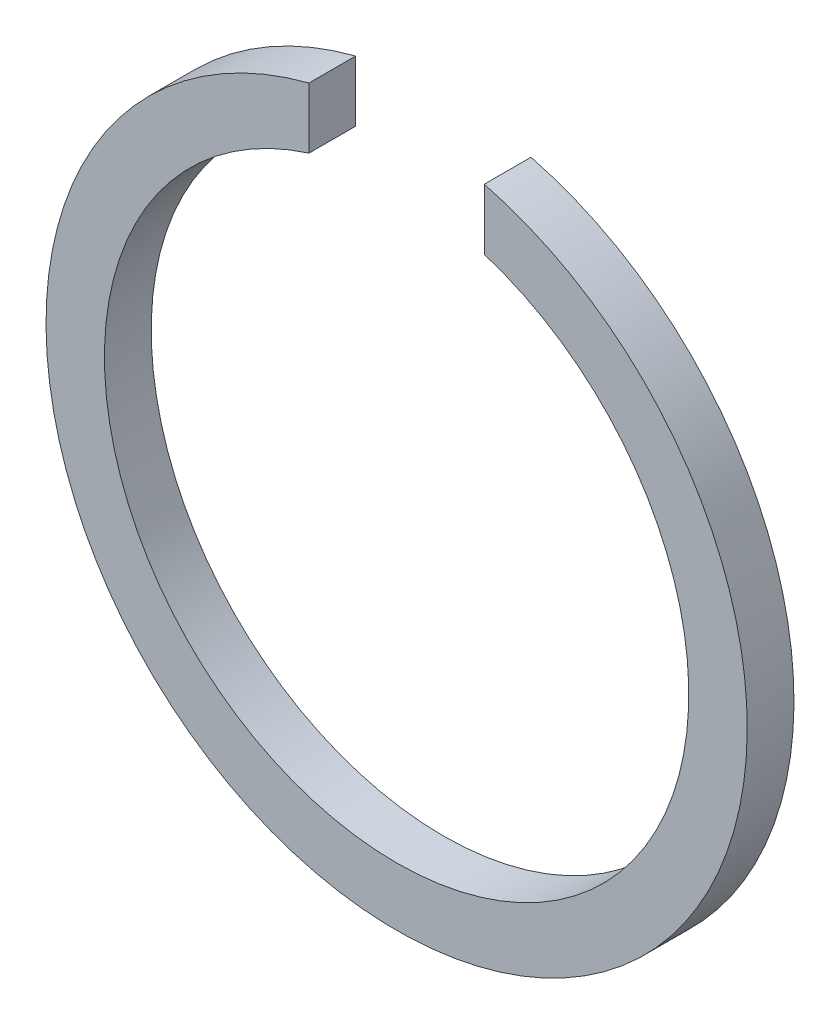
from build123d import *

# Parameters (mm, degrees)
SKETCH1_R           = 60
SKETCH1_R_2         = 50
BOSS_EXTRUDE1_DEPTH = 8
SKETCH2_W           = 30
SKETCH2_H           = 71.834610917
CUT_EXTRUDE1_DEPTH  = 15


with BuildPart() as part:
    # Sketch1 → Boss-Extrude1 (new body)
    with BuildSketch(Plane.XY):
        Circle(SKETCH1_R)
        Circle(SKETCH1_R_2, mode=Mode.SUBTRACT)
    extrude(amount=BOSS_EXTRUDE1_DEPTH)

    # Sketch2 → Cut-Extrude1 (cut)
    with BuildSketch(Plane.XY.offset(8)):
        with Locations((0, 51.497328688)):
            Rectangle(SKETCH2_W, SKETCH2_H)
    extrude(amount=-CUT_EXTRUDE1_DEPTH, mode=Mode.SUBTRACT)


solid = part.part
